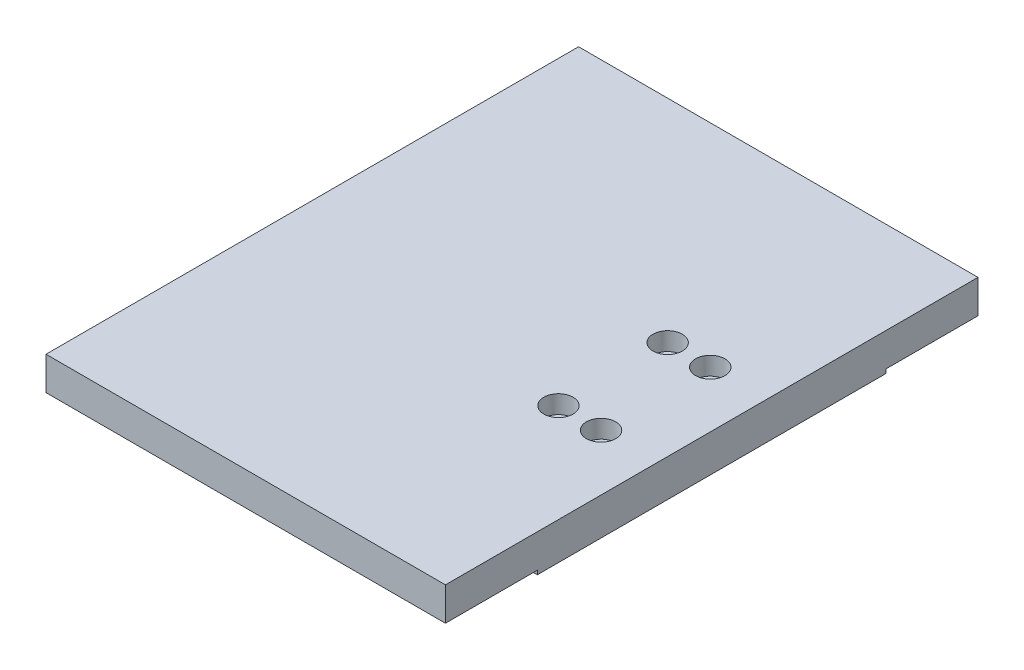
from build123d import *

# Parameters (mm, degrees)
SKETCH_1_W                = 150
SKETCH_1_H                = 200
EXTRUDE_1_DEPTH           = 14
SKETCH_2_W                = 150
SKETCH_2_H                = 34.5
CUT_EXTRUDE_1_DEPTH       = 1.5
HOLE_WIZARD_1_D           = 6.6
HOLE_WIZARD_1_CBORE_D     = 11
HOLE_WIZARD_1_CBORE_DEPTH = 6.8


with BuildPart() as part:
    # 草图1 → 凸台-拉伸1 (new body)
    with BuildSketch(Plane(origin=(0, 0, 0), x_dir=(1, 0, 0), z_dir=(0, 1, 0))):
        Rectangle(SKETCH_1_W, SKETCH_1_H)
    extrude(amount=EXTRUDE_1_DEPTH)

    # 草图2 → 切除-拉伸1 (cut)
    with BuildSketch(Plane.XZ):
        with Locations((0, 82.75)):
            Rectangle(SKETCH_2_W, SKETCH_2_H)
        with Locations((0, -82.75)):
            Rectangle(SKETCH_2_W, SKETCH_2_H)
    extrude(amount=-CUT_EXTRUDE_1_DEPTH, mode=Mode.SUBTRACT)

    # 打孔尺寸(%根据)内六角圆柱头螺钉的类型1 (through all)
    with Locations(Plane(origin=(37.95, 14, 20.5), x_dir=(0, 0, 1), z_dir=(0, 1, 0))):
        with Locations((0, 0), (-41, 0), (0, 16), (-41, 16)):
            CounterBoreHole(HOLE_WIZARD_1_D / 2, HOLE_WIZARD_1_CBORE_D / 2, HOLE_WIZARD_1_CBORE_DEPTH)


solid = part.part
